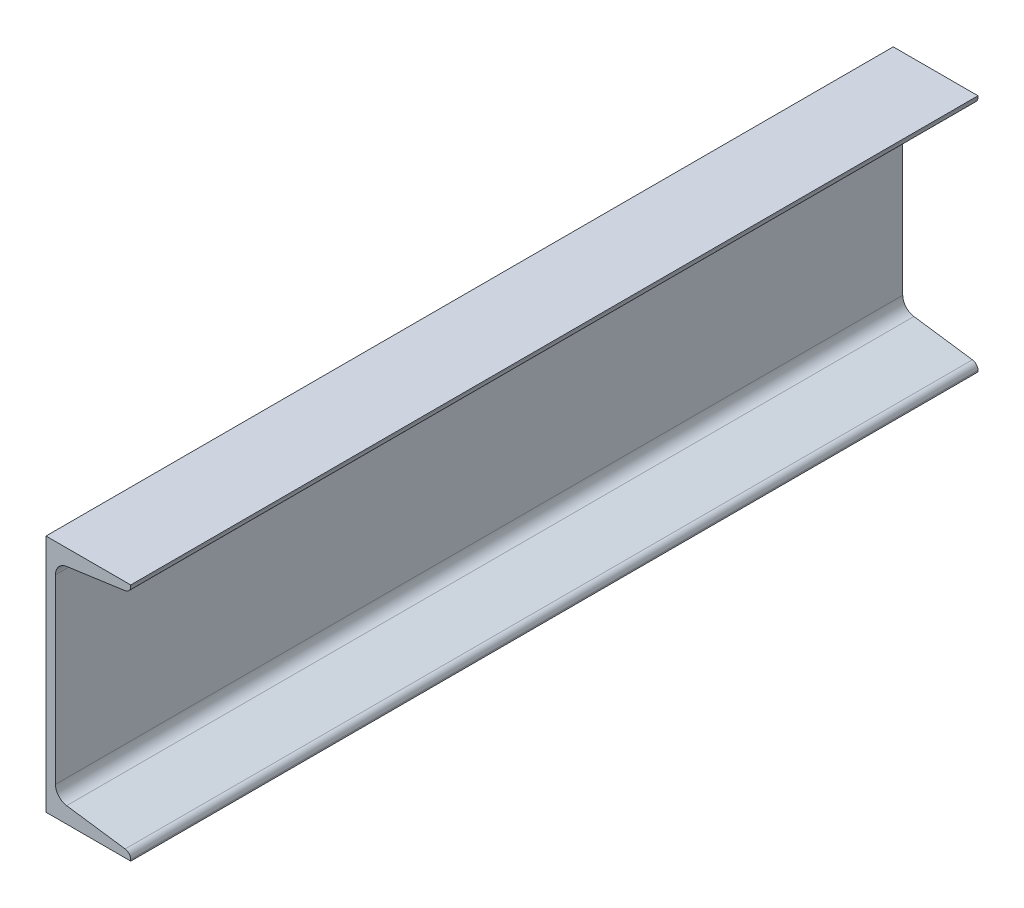
from build123d import *

# Parameters (mm, degrees)
EXTRUDE_1_DEPTH = 850


with BuildPart() as part:
    # 草图1 → 凸台-拉伸1 (new body)
    with BuildSketch(Plane.XY):
        with BuildLine():
            Line((0, 0), (-85, 0))
            Line((-85, 0), (-85, -240))
            Line((-85, -240), (0, -240))
            Line((0, -240), (0, -238.623349271))
            ThreePointArc((0, -238.623349271), (-1.594387729, -234.358965582), (-5.595374844, -232.186606824))
            Line((-5.595374844, -232.186606824), (-64.309250312, -223.934909757))
            ThreePointArc((-64.309250312, -223.934909757), (-72.311224543, -219.59019224), (-75.5, -211.061424863))
            Line((-75.5, -211.061424863), (-75.5, -28.938575137))
            ThreePointArc((-75.5, -28.938575137), (-72.311224543, -20.40980776), (-64.309250312, -16.065090243))
            Line((-64.309250312, -16.065090243), (-5.595374844, -7.813393176))
            ThreePointArc((-5.595374844, -7.813393176), (-1.594387729, -5.641034418), (0, -1.376650729))
            Line((0, -1.376650729), (0, 0))
        make_face()
    extrude(amount=EXTRUDE_1_DEPTH)


solid = part.part
